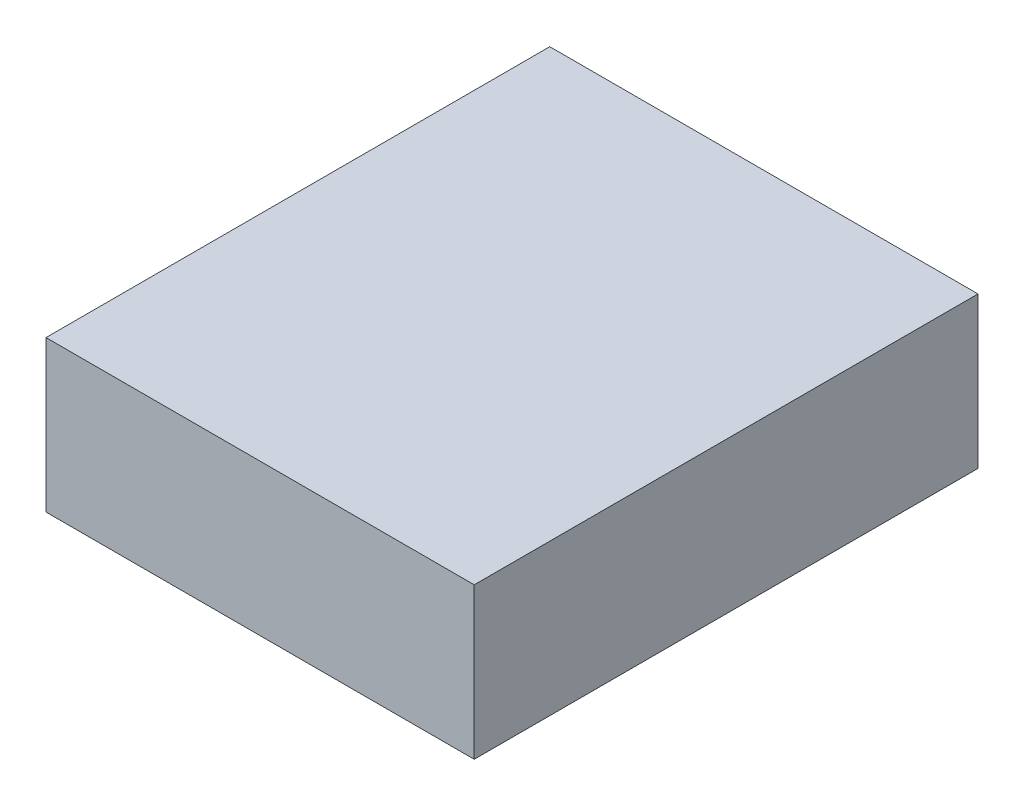
from build123d import *

# Parameters (mm, degrees)
SKETCH1_W           = 100
SKETCH1_H           = 30
BOSS_EXTRUDE1_DEPTH = 85


with BuildPart() as part:
    # Sketch1 → Boss-Extrude1 (new body)
    with BuildSketch(Plane(origin=(0, 0, 0), x_dir=(0, 0, -1), z_dir=(1, 0, 0))):
        with Locations((50, 15)):
            Rectangle(SKETCH1_W, SKETCH1_H)
    extrude(amount=BOSS_EXTRUDE1_DEPTH)


solid = part.part
